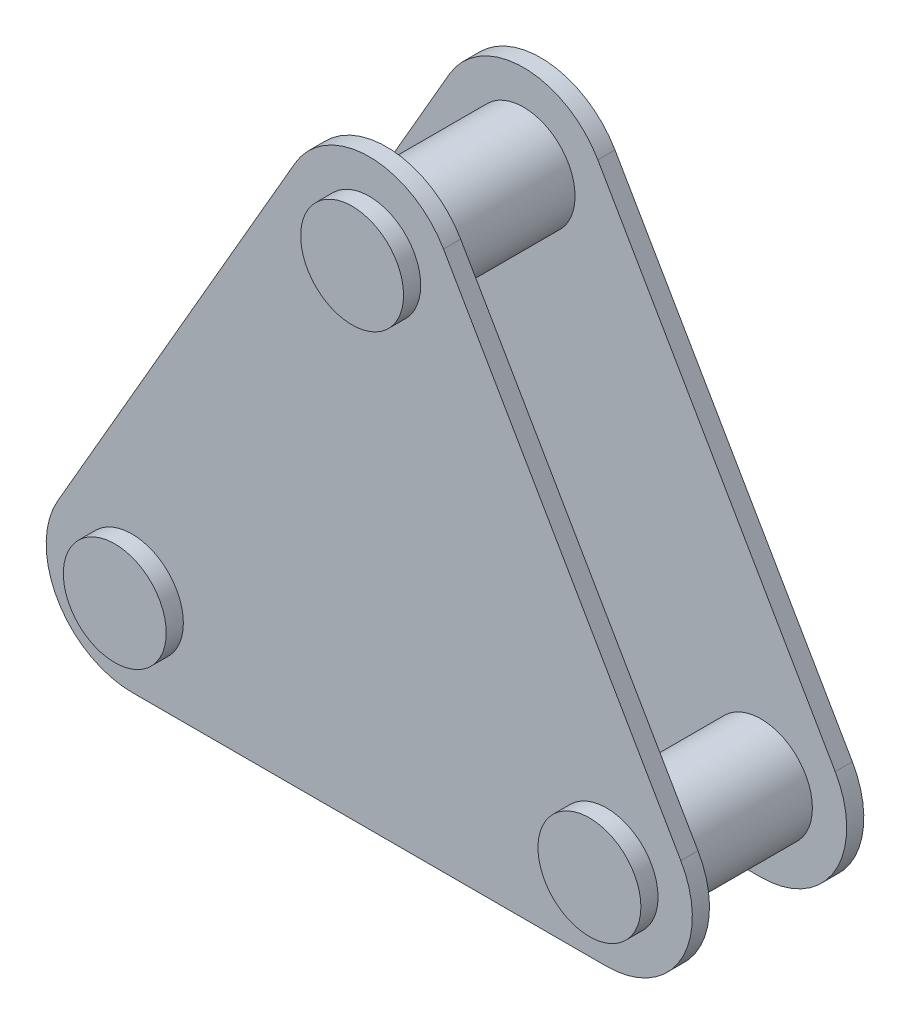
from build123d import *

# Parameters (mm, degrees)
SKETCH1_R           = 3
BOSS_EXTRUDE1_DEPTH = 1
BOSS_EXTRUDE2_START = -11
SKETCH2_R           = 3
BOSS_EXTRUDE2_DEPTH = 11
SKETCH3_R           = 3
BOSS_EXTRUDE3_DEPTH = 1


with BuildPart() as part:
    # Sketch1 → Boss-Extrude1 (new body)
    with BuildSketch(Plane.XY):
        with BuildLine():
            Line((18.169872981, -5.490381057), (4.330127019, 18.480762114))
            ThreePointArc((4.330127019, 18.480762114), (0, 20.980762114), (-4.330127019, 18.480762114))
            Line((-4.330127019, 18.480762114), (-18.169872981, -5.490381057))
            ThreePointArc((-18.169872981, -5.490381057), (-18.169872981, -10.490381057), (-13.839745962, -12.990381057))
            Line((-13.839745962, -12.990381057), (13.839745962, -12.990381057))
            ThreePointArc((13.839745962, -12.990381057), (18.169872981, -10.490381057), (18.169872981, -5.490381057))
        make_face()
        with Locations((0, 15.980762114)):
            Circle(SKETCH1_R, mode=Mode.SUBTRACT)
        with Locations((13.839745962, -7.990381057)):
            Circle(SKETCH1_R, mode=Mode.SUBTRACT)
        with Locations((-13.839745962, -7.990381057)):
            Circle(SKETCH1_R, mode=Mode.SUBTRACT)
    boss_extrude1 = extrude(amount=BOSS_EXTRUDE1_DEPTH)

    # Sketch2 → Boss-Extrude2 (add)
    with BuildSketch(Plane.XY.offset(1).offset(BOSS_EXTRUDE2_START)):
        with Locations((13.839745962, -7.990381057)):
            Circle(SKETCH2_R)
        with Locations((-13.839745962, -7.990381057)):
            Circle(SKETCH2_R)
        with Locations((0, 15.980762114)):
            Circle(SKETCH2_R)
    extrude(amount=BOSS_EXTRUDE2_DEPTH)

    # Mirror3: Boss-Extrude1 across plane
    add(boss_extrude1.mirror(Plane(origin=(0, 0, -4), x_dir=(1, 0, 0), z_dir=(0, 0, -1))))

    # Sketch3 → Boss-Extrude3 (add)
    with BuildSketch(Plane.XY.offset(1)):
        with Locations((0, 15.980762114)):
            Circle(SKETCH3_R)
        with Locations((13.839745962, -7.990381057)):
            Circle(SKETCH3_R)
        with Locations((-13.839745962, -7.990381057)):
            Circle(SKETCH3_R)
    extrude(amount=BOSS_EXTRUDE3_DEPTH)


solid = part.part
